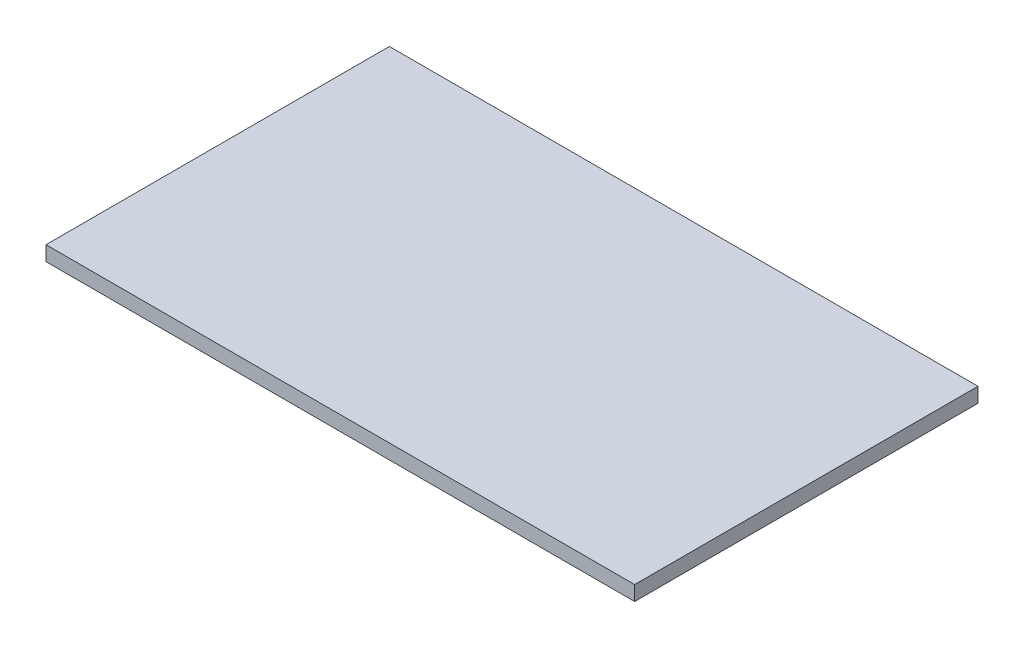
from build123d import *

# Parameters (mm, degrees)
SKETCH_1_W      = 120
SKETCH_1_H      = 3
EXTRUDE_1_DEPTH = 70


with BuildPart() as part:
    # 草图1 → 凸台-拉伸1 (new body)
    with BuildSketch(Plane.XY):
        Rectangle(SKETCH_1_W, SKETCH_1_H)
    extrude(amount=EXTRUDE_1_DEPTH)


solid = part.part
